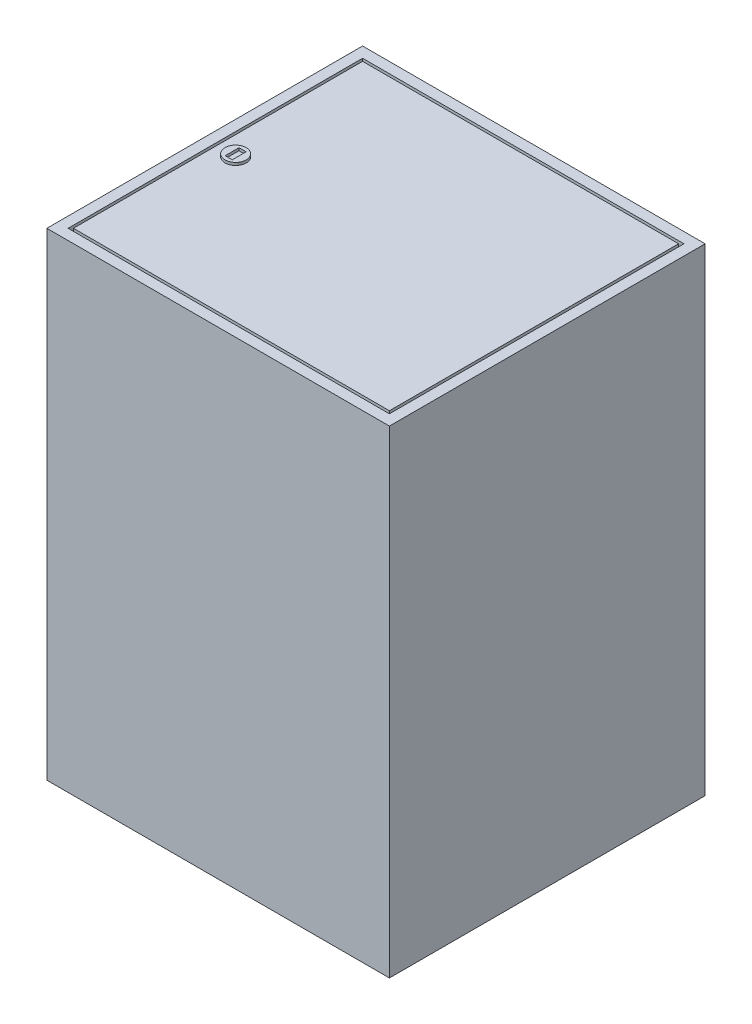
SolidWorks part; units mm, degrees
ref_plane "前视基准面" through (0, 0, 0) normal (0, 0, 1) x (1, 0, 0)
ref_plane "上视基准面" through (0, 0, 0) normal (0, 1, 0) x (1, 0, 0)
ref_plane "右视基准面" through (0, 0, 0) normal (1, 0, 0) x (0, 0, -1)
sketch "草图1" plane through (0, 0, 0) normal (0, 0, 1) x (1, 0, 0)
  line L1 (-322.5, 450) -> (322.5, 450)
  line L2 (-322.5, 450) -> (-322.5, -450)
  line L3 (-322.5, -450) -> (322.5, -450)
  line L4 (322.5, 450) -> (322.5, -450)
  line L5 (-322.5, 450) -> (322.5, -450) construction
  line L6 (-322.5, -450) -> (322.5, 450) construction
  point P0 (0, 0)
  dimension "D1" = 900
  dimension "D2" = 645
extrude "凸台-拉伸1" add sketch "草图1" along normal blind 594.5
sketch "草图2" plane through (0, -450, 0) normal (0, -1, 0) x (1, 0, 0)
  line L0 (-322.5, 0) -> (322.5, 0) construction
  line L1 (-302.5, 574.5) -> (302.5, 574.5)
  line L2 (-302.5, 574.5) -> (-302.5, 20)
  line L3 (-302.5, 20) -> (302.5, 20)
  line L4 (302.5, 574.5) -> (302.5, 20)
  line L5 (-302.5, 574.5) -> (302.5, 20) construction
  line L6 (-302.5, 20) -> (302.5, 574.5) construction
  line L7 (322.5, 594.5) -> (322.5, 0) construction
  line L8 (-322.5, 594.5) -> (-322.5, 0) construction
  line L9 (-322.5, 594.5) -> (322.5, 594.5) construction
  line L10 (-297.5, 25) -> (297.5, 25)
  line L11 (297.5, 569.5) -> (297.5, 25)
  line L12 (-297.5, 569.5) -> (297.5, 569.5)
  line L13 (-297.5, 569.5) -> (-297.5, 25)
  point P0 (0, 297.25)
  dimension "D1" = 20
  dimension "D2" = 20
  dimension "D3" = 20
  dimension "D4" = 20
  dimension "D5" = 5
extrude "切除-拉伸1" cut sketch "草图2" against normal blind 10
sketch "草图3" plane through (0, -450, 0) normal (0, -1, 0) x (1, 0, 0)
  circle A0 centre (263.5923, 304.2299) radius 20
  dimension "D1" = 40
extrude "凸台-拉伸2" add sketch "草图3" along normal blind 5
sketch "草图4" plane through (0, -455, 0) normal (0, -1, 0) x (1, 0, 0)
  line L1 (268.5576, 316.5597) -> (258.627, 316.5597)
  line L2 (268.5576, 316.5597) -> (268.5576, 291.9001)
  line L3 (268.5576, 291.9001) -> (258.627, 291.9001)
  line L4 (258.627, 316.5597) -> (258.627, 291.9001)
  line L5 (268.5576, 316.5597) -> (258.627, 291.9001) construction
  line L6 (268.5576, 291.9001) -> (258.627, 316.5597) construction
  point P0 (263.5923, 304.2299)
extrude "切除-拉伸2" cut sketch "草图4" against normal blind 5
sketch "草图5" plane through (0, 450, 0) normal (0, 1, 0) x (1, 0, 0)
  line L4 (-302.5, -574.5) -> (302.5, -574.5)
  line L5 (302.5, -574.5) -> (302.5, -20)
  line L6 (302.5, -20) -> (-302.5, -20)
  line L7 (-302.5, -20) -> (-302.5, -574.5)
  line L8 (-302.5, -574.5) -> (302.5, -574.5)
  line L9 (302.5, -574.5) -> (302.5, -20)
  line L10 (302.5, -20) -> (-302.5, -20)
  line L11 (-302.5, -20) -> (-302.5, -574.5)
  line L12 (-297.5, -569.5) -> (297.5, -569.5)
  line L13 (-297.5, -25) -> (-297.5, -569.5)
  line L14 (297.5, -25) -> (-297.5, -25)
  line L15 (297.5, -569.5) -> (297.5, -25)
  line L16 (-297.5, -569.5) -> (297.5, -569.5)
  line L17 (-297.5, -25) -> (-297.5, -569.5)
  line L18 (297.5, -25) -> (-297.5, -25)
  line L19 (297.5, -569.5) -> (297.5, -25)
  dimension "D1" = 0
  dimension "D2" = 0
extrude "切除-拉伸3" cut sketch "草图5" against normal blind 10
sketch "草图6" plane through (0, 450, 0) normal (0, 1, 0) x (1, 0, 0)
  circle A0 centre (-261.3259, -300.2062) radius 20
  dimension "D1" = 40
extrude "凸台-拉伸3" add sketch "草图6" along normal blind 5
sketch "草图7" plane through (0, 455, 0) normal (0, 1, 0) x (1, 0, 0)
  line L1 (-254.6334, -313.239) -> (-268.0185, -313.239)
  line L2 (-254.6334, -313.239) -> (-254.6334, -287.1733)
  line L3 (-254.6334, -287.1733) -> (-268.0185, -287.1733)
  line L4 (-268.0185, -313.239) -> (-268.0185, -287.1733)
  line L5 (-254.6334, -313.239) -> (-268.0185, -287.1733) construction
  line L6 (-254.6334, -287.1733) -> (-268.0185, -313.239) construction
  point P0 (-261.3259, -300.2062)
extrude "切除-拉伸4" cut sketch "草图7" against normal blind 5
